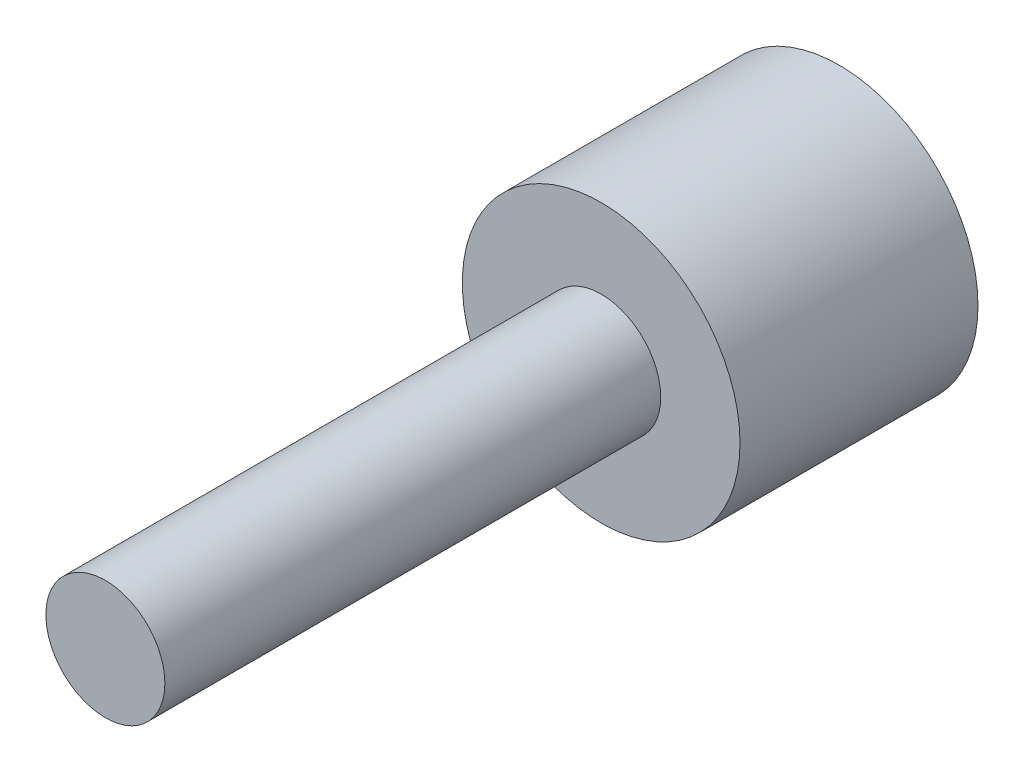
from build123d import *

# Parameters (mm, degrees)
SKETCH_1_R      = 7
EXTRUDE_1_DEPTH = 12
SKETCH_2_R      = 3
EXTRUDE_2_DEPTH = 25


with BuildPart() as part:
    # 草图1 → 凸台-拉伸1 (new body)
    with BuildSketch(Plane.XY):
        Circle(SKETCH_1_R)
    extrude(amount=EXTRUDE_1_DEPTH)

    # 草图2 → 凸台-拉伸2 (add)
    with BuildSketch(Plane.XY.offset(12)):
        Circle(SKETCH_2_R)
    extrude(amount=EXTRUDE_2_DEPTH)


solid = part.part
